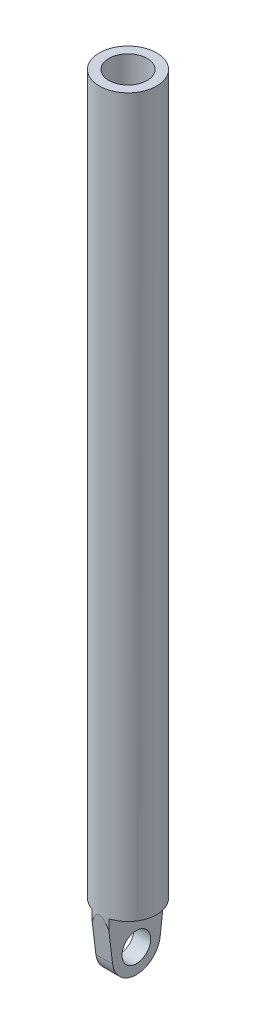
SolidWorks part; units mm, degrees
ref_plane "Front Plane" through (0, 0, 0) normal (0, 0, 1) x (1, 0, 0)
ref_plane "Top Plane" through (0, 0, 0) normal (0, 1, 0) x (1, 0, 0)
ref_plane "Right Plane" through (0, 0, 0) normal (1, 0, 0) x (0, 0, -1)
sketch "Sketch1" plane through (0, 0, 0) normal (0, 1, 0) x (1, 0, 0)
  circle A0 centre (0, 0) radius 6
  dimension "D1" = 12
extrude "Boss-Extrude1" add sketch "Sketch1" along normal blind 150
shell "Shell1" thickness 2
sketch "Sketch2" plane through (0, 0, 0) normal (1, 0, 0) x (0, 0, -1)
  line L0 (-6, 0) -> (6, 0)
  line L1 (-6, 0) -> (-4.9641, -8.5981)
  line L2 (6, 0) -> (4.9641, -8.5981)
  circle A0 centre (0, -8) radius 3
  arc A1 (-4.9641, -8.5981) -> (4.9641, -8.5981) centre (0, -8) ccw
  dimension "D1" = 6
  dimension "D2" = 10
  dimension "D3" = 8
extrude "Boss-Extrude2" add sketch "Sketch2" along normal mid plane 3.5
sketch "Sketch3" plane through (0, 0, 0) normal (0, -1, 0) x (1, 0, 0)
  circle A0 centre (0, 0) radius 6
  circle A1 centre (0, 0) radius 8.5782
extrude "Cut-Extrude1" cut sketch "Sketch3" along normal blind 10
